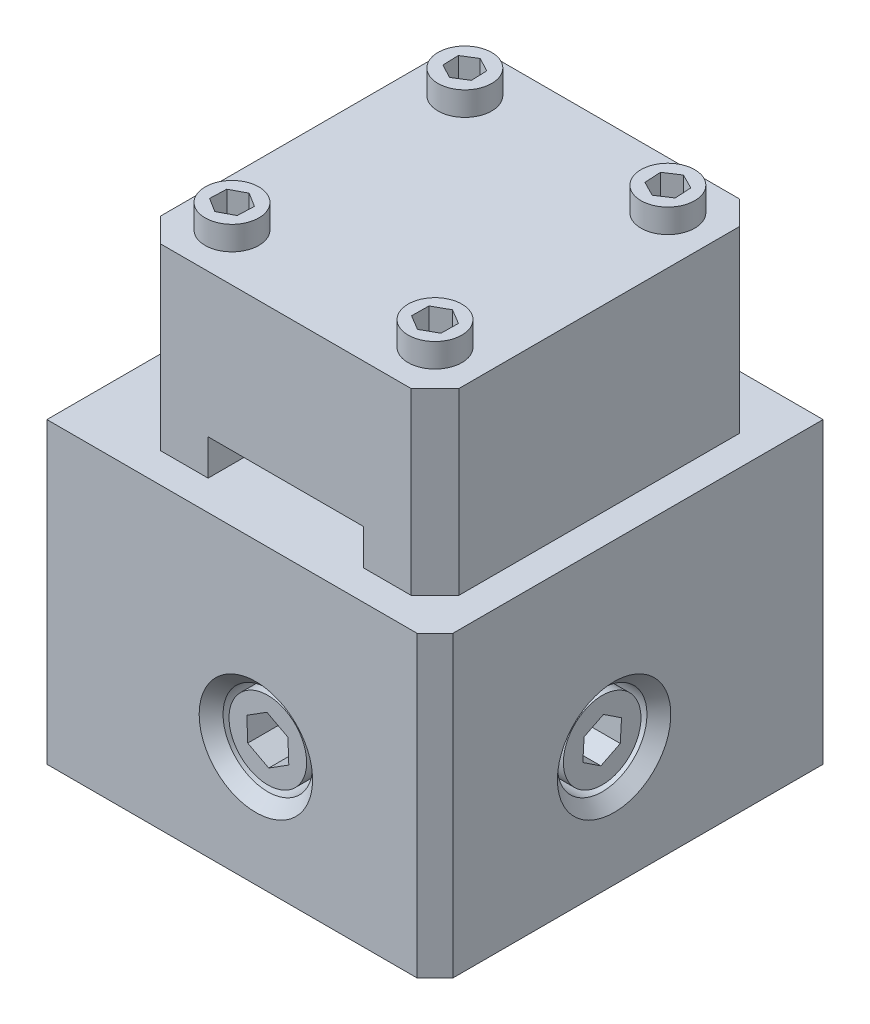
SolidWorks part; units mm, degrees
ref_plane "Front Plane" through (0, 0, 0) normal (0, 0, 1) x (1, 0, 0)
ref_plane "Top Plane" through (0, 0, 0) normal (0, 1, 0) x (1, 0, 0)
ref_plane "Right Plane" through (0, 0, 0) normal (1, 0, 0) x (0, 0, -1)
other "Configuration Table"
sketch "Sketch1" plane through (0, 0, 0) normal (0, 1, 0) x (1, 0, 0)
  line L0 (20, 20) -> (20, 35)
  line L5 (-20, 20) -> (20, 20)
  line L7 (-20, 20) -> (-20, -20)
  line L8 (-20, -20) -> (20, -20) construction
  line L9 (20, 20) -> (20, -20) construction
  line L10 (-20, 20) -> (20, -20) construction
  line L11 (-20, -20) -> (20, 20) construction
  line L12 (20, 35) -> (30, 35)
  line L13 (30, 35) -> (30, -30)
  line L14 (30, -30) -> (-35, -30)
  line L15 (-35, -30) -> (-35, -20)
  line L16 (-35, -20) -> (-20, -20)
  point P0 (0, 0)
  dimension "D1" = 40
  dimension "D2" = 40
  dimension "D3" = 10
  dimension "D4" = 10
  dimension "D5" = 15
  dimension "D6" = 15
extrude "Boss-Extrude1" add sketch "Sketch1" along normal blind 40
sketch "Sketch3" plane through (0, 40, 0) normal (0, 1, 0) x (1, 0, 0)
  line L1 (30, -30) -> (-35, -30)
  line L2 (30, -30) -> (30, 35)
  line L3 (30, 35) -> (-35, 35)
  line L4 (-35, -30) -> (-35, 35)
  dimension "D1" = 65
  dimension "D2" = 65
extrude "Boss-Extrude3" add sketch "Sketch3" along normal blind 10
sketch "Sketch4" plane through (0, 0, 30) normal (0, 0, 1) x (1, 0, 0)
  line L0 (30, 50) -> (30, 0) construction
  line L1 (-35, 0) -> (30, 0) construction
  circle A0 centre (0, 20) radius 7.5
  dimension "D1" = 15
  dimension "D2" = 30
  dimension "D3" = 20
extrude "Cut-Extrude1" cut sketch "Sketch4" against normal blind 10
sketch "Sketch5" plane through (30, 0, 0) normal (1, 0, 0) x (0, 0, -1)
  line L0 (-30, 50) -> (-30, 0) construction
  line L1 (-30, 0) -> (35, 0) construction
  circle A0 centre (0, 20) radius 7.5
  dimension "D1" = 15
  dimension "D2" = 30
  dimension "D3" = 20
extrude "Cut-Extrude2" cut sketch "Sketch5" against normal blind 10
sketch "Sketch6" plane through (0, 0, 20) normal (0, 0, 1) x (1, 0, 0)
  line L1 (3.513, 18.143) -> (3.3647, 22.1139)
  line L2 (3.3647, 22.1139) -> (-0.1483, 23.9709)
  line L3 (-0.1483, 23.9709) -> (-3.513, 21.857)
  line L4 (-3.513, 21.857) -> (-3.3647, 17.8861)
  line L5 (-3.3647, 17.8861) -> (0.1483, 16.0291)
  line L6 (0.1483, 16.0291) -> (3.513, 18.143)
  circle A0 centre (0, 20) radius 6.5
  circle A1 centre (0, 20) radius 3.4413 construction
  dimension "D1" = 13
extrude "Boss-Extrude4" add sketch "Sketch6" along normal blind 8
sketch "Sketch7" plane through (20, 0, 0) normal (1, 0, 0) x (0, 0, -1)
  line L1 (3.0275, 18.0024) -> (3.2437, 21.623)
  line L2 (3.2437, 21.623) -> (0.2163, 23.6207)
  line L3 (0.2163, 23.6207) -> (-3.0275, 21.9976)
  line L4 (-3.0275, 21.9976) -> (-3.2437, 18.377)
  line L5 (-3.2437, 18.377) -> (-0.2163, 16.3793)
  line L6 (-0.2163, 16.3793) -> (3.0275, 18.0024)
  circle A0 centre (0, 20) radius 6.5
  circle A1 centre (0, 20) radius 3.1412 construction
  dimension "D1" = 13
extrude "Boss-Extrude5" add sketch "Sketch7" along normal blind 8
chamfer "Chamfer1" distance 2 angle 45 2 edges at (7.5, 20, 30) (30, 20, -7.5)
chamfer "Chamfer2" distance 3 angle 45 1 edges at (30, 25, 30)
sketch "Sketch9" plane through (30, 0, 0) normal (1, 0, 0) x (0, 0, -1)
  line L0 (-25, 50) -> (-25, 80)
  line L1 (-27, 50) -> (35, 50) construction
  line L2 (-25, 80) -> (30, 80)
  line L3 (30, 80) -> (30, 50)
  line L4 (30, 50) -> (20, 50)
  line L5 (20, 50) -> (20, 75)
  line L6 (20, 75) -> (-15, 75)
  line L7 (-15, 75) -> (-15, 50)
  line L8 (-15, 50) -> (-25, 50)
  line L9 (35, 50) -> (35, 0) construction
  line L10 (-30, 0) -> (-30, 50) construction
  dimension "D1" = 5
  dimension "D2" = 5
  dimension "D3" = 10
  dimension "D4" = 10
  dimension "D5" = 30
  dimension "D6" = 25
extrude "Boss-Extrude6" add sketch "Sketch9" against normal blind 55
sketch "Sketch10" plane through (30, 0, 0) normal (1, 0, 0) x (0, 0, -1)
  line L1 (-25, 80) -> (30, 80)
  line L2 (-25, 80) -> (-25, 50)
  line L3 (-25, 50) -> (30, 50)
  line L4 (30, 80) -> (30, 50)
extrude "Cut-Extrude3" cut sketch "Sketch10" against normal blind 5
sketch "Sketch12" plane through (25, 0, 0) normal (1, 0, 0) x (0, 0, -1)
  line L1 (-17.9429, 76.013) -> (22.9429, 76.013)
  line L2 (-17.9429, 76.013) -> (-17.9429, 45.4328)
  line L3 (-17.9429, 45.4328) -> (22.9429, 45.4328)
  line L4 (22.9429, 76.013) -> (22.9429, 45.4328)
extrude "Boss-Extrude10" add sketch "Sketch12" against normal blind 5
sketch "Sketch13" plane through (0, 0, 25) normal (0, 0, 1) x (1, 0, 0)
  line L0 (30, 50) -> (-35, 50) construction
  line L1 (-13, 50) -> (13, 50)
  line L2 (-13, 50) -> (-13, 56)
  line L3 (-13, 56) -> (13, 56)
  line L4 (13, 50) -> (13, 56)
  line L5 (25, 80) -> (25, 50) construction
  line L6 (-25, 80) -> (-25, 50) construction
  dimension "D1" = 12
  dimension "D2" = 6
  dimension "D3" = 12
extrude "Cut-Extrude4" cut sketch "Sketch13" against normal blind 65
sketch "Sketch14" plane through (0, 80, 0) normal (0, 1, 0) x (1, 0, 0)
  line L0 (-25, 30) -> (25, 30) construction
  line L1 (-17, 22) -> (17, 22) construction
  line L2 (-17, 22) -> (-17, -17) construction
  line L3 (-17, -17) -> (17, -17) construction
  line L4 (17, 22) -> (17, -17) construction
  line L5 (-25, 30) -> (-25, -25) construction
  line L6 (25, 30) -> (25, -25) construction
  line L7 (-25, -25) -> (25, -25) construction
  line L9 (-14.6502, 20.748) -> (-14.7409, 23.409)
  line L10 (-14.7409, 23.409) -> (-17.0907, 24.661)
  line L11 (-17.0907, 24.661) -> (-19.3498, 23.252)
  line L12 (-19.3498, 23.252) -> (-19.2591, 20.591)
  line L13 (-19.2591, 20.591) -> (-16.9093, 19.339)
  line L14 (-16.9093, 19.339) -> (-14.6502, 20.748)
  line L15 (19.4796, 20.748) -> (19.324, 23.5214)
  line L16 (19.324, 23.5214) -> (16.8444, 24.7733)
  line L17 (16.8444, 24.7733) -> (14.5204, 23.252)
  line L18 (14.5204, 23.252) -> (14.676, 20.4786)
  line L19 (14.676, 20.4786) -> (17.1556, 19.2267)
  line L20 (17.1556, 19.2267) -> (19.4796, 20.748)
  line L21 (-14.6502, -18.4784) -> (-14.5447, -15.7042)
  line L22 (-14.5447, -15.7042) -> (-16.8945, -14.2258)
  line L23 (-16.8945, -14.2258) -> (-19.3498, -15.5216)
  line L24 (-19.3498, -15.5216) -> (-19.4553, -18.2958)
  line L25 (-19.4553, -18.2958) -> (-17.1055, -19.7742)
  line L26 (-17.1055, -19.7742) -> (-14.6502, -18.4784)
  line L27 (19.4796, -18.4784) -> (19.5201, -15.5918)
  line L28 (19.5201, -15.5918) -> (17.0406, -14.1134)
  line L29 (17.0406, -14.1134) -> (14.5204, -15.5216)
  line L30 (14.5204, -15.5216) -> (14.4799, -18.4082)
  line L31 (14.4799, -18.4082) -> (16.9594, -19.8866)
  line L32 (16.9594, -19.8866) -> (19.4796, -18.4784)
  circle A0 centre (-17, 22) radius 4.5
  circle A1 centre (17, 22) radius 4.5
  circle A2 centre (17, -17) radius 4.5
  circle A3 centre (-17, -17) radius 4.5
  circle A4 centre (-17, 22) radius 2.3058 construction
  circle A5 centre (17, 22) radius 2.4056 construction
  circle A6 centre (-17, -17) radius 2.4043 construction
  circle A7 centre (17, -17) radius 2.5001 construction
  dimension "D5" = 9
  dimension "D1" = 8
  dimension "D2" = 8
  dimension "D3" = 8
  dimension "D4" = 8
extrude "Boss-Extrude11" add sketch "Sketch14" along normal blind 4
chamfer "Chamfer3" distance 4 angle 45 4 edges at (25, 65, -30) (25, 65, 25) (-25, 65, 25) (-25, 65, -30)
